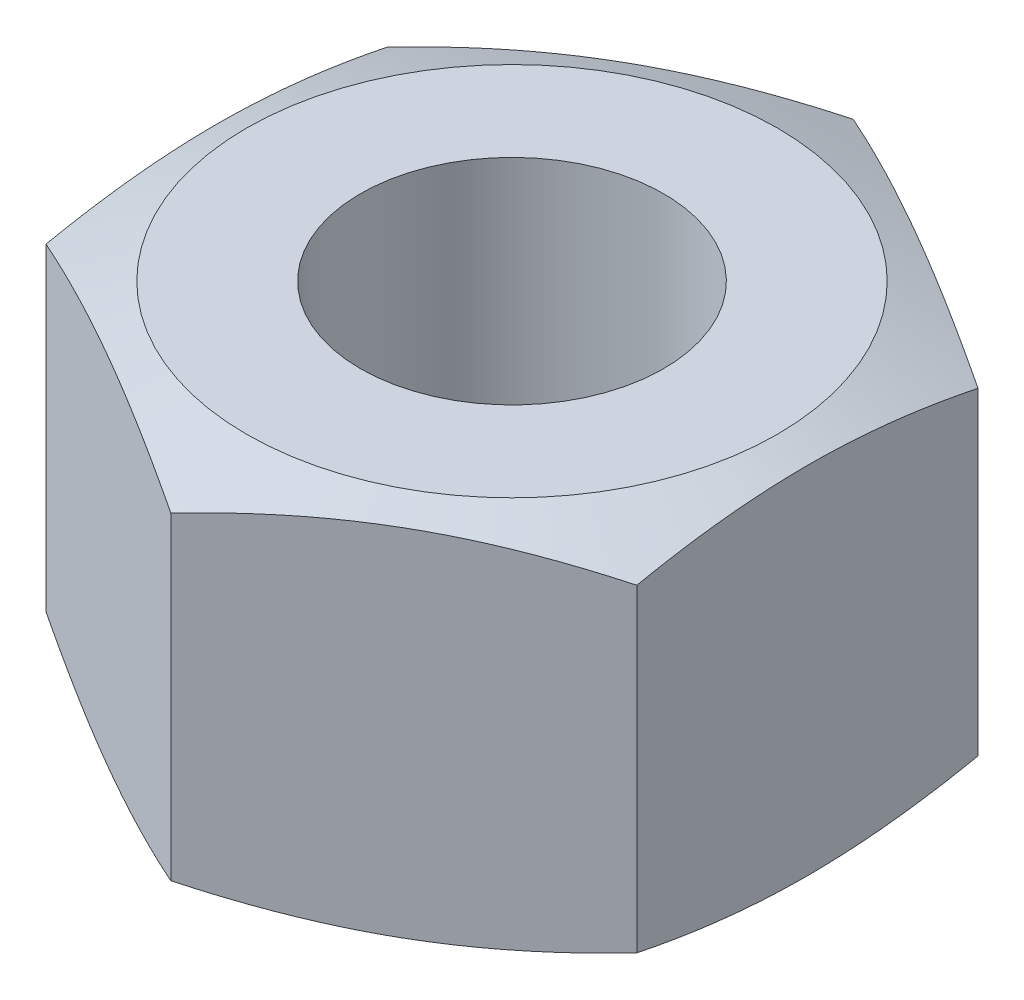
from build123d import *

# Parameters (mm, degrees)
SKETCH_1_R      = 10
EXTRUDE_1_DEPTH = 12.5


with BuildPart() as part:
    # 草图1 → 凸台-拉伸1 (new, symmetric)
    with BuildSketch(Plane(origin=(0, 0, 0), x_dir=(1, 0, 0), z_dir=(0, 1, 0))):
        Polygon((0, 22.5), (-19.485571585, 11.25), (-19.485571585, -11.25), (0, -22.5), (19.485571585, -11.25), (19.485571585, 11.25), align=None)
        with Locations(Location((0, 0, 0), (0, 0, 270))):
            Circle(SKETCH_1_R, mode=Mode.SUBTRACT)
    extrude(amount=EXTRUDE_1_DEPTH, both=True)

    # 草图2 → 切除-旋转1 (revolve, cut)
    with BuildSketch(Plane(origin=(0, 0, 0), x_dir=(0, 0, -1), z_dir=(1, 0, 0))):
        with BuildLine():
            Line((-22.5, 10.5), (-22.5, 12.5))
            Line((-22.5, 12.5), (-17.5, 12.5))
            ThreePointArc((-17.5, 12.5), (-20.005385321, 11.513463302), (-22.5, 10.5))
        make_face()
    cut_revolve_1 = revolve(axis=Axis((0, 32.499694269, 0), (0, -1, 0)), mode=Mode.SUBTRACT)

    # 镜向1: 切除-旋转1 across plane
    add(cut_revolve_1.mirror(Plane.ZX), mode=Mode.SUBTRACT)


solid = part.part
